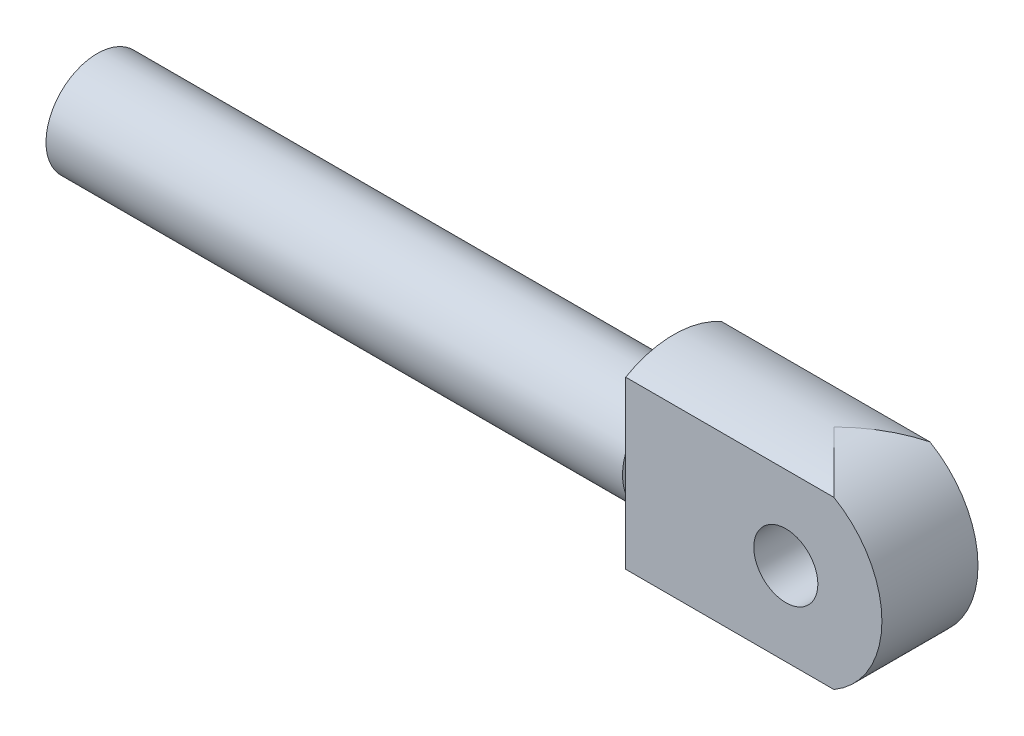
from build123d import *

# Parameters (mm, degrees)
BOSS_EXTRUDE1_START     = 100
SKETCH1_R               = 80
SKETCH1_R_2             = 50
BOSS_EXTRUDE1_DEPTH     = 900
BOSS_EXTRUDE2_DEPTH     = 400
CUT_EXTRUDE2_DEPTH      = 1417.518619715
CUT_EXTRUDE2_DEPTH_BACK = 1417.518619715
CUT_EXTRUDE3_DEPTH      = 1417.518619715
CUT_EXTRUDE3_DEPTH_BACK = 1417.518619715
SKETCH_4_5_2_R          = 50


with BuildPart() as part:
    # Sketch1 → Boss-Extrude1 (new body)
    with BuildSketch(Plane(origin=(0, 0, 0), x_dir=(0, 0, -1), z_dir=(1, 0, 0)).offset(BOSS_EXTRUDE1_START)):
        Circle(SKETCH1_R)
        Circle(SKETCH1_R_2, mode=Mode.SUBTRACT)
    extrude(amount=BOSS_EXTRUDE1_DEPTH)

    # Sketch3 → Boss-Extrude2 (add)
    with BuildSketch(Plane(origin=(1000, 0, 0), x_dir=(0, 0, -1), z_dir=(1, 0, 0))):
        with BuildLine():
            Line((-75, 129.903810568), (-75, -129.903810568))
            ThreePointArc((-75, -129.903810568), (0, -150), (75, -129.903810568))
            Line((75, -129.903810568), (75, 129.903810568))
            ThreePointArc((75, 129.903810568), (0, 150), (-75, 129.903810568))
        make_face()
    extrude(amount=BOSS_EXTRUDE2_DEPTH)

    # Sketch 4_5 → Cut-Extrude2 (cut, two sides: drawn at the far end of the back side and taken through both)
    with BuildSketch(Plane.XY.offset(75).offset(-CUT_EXTRUDE2_DEPTH_BACK)):
        with BuildLine():
            Line((1250, 150), (1455.357524725, 150))
            Line((1455.357524725, 150), (1455.357524725, -150))
            Line((1455.357524725, -150), (1250, -150))
            ThreePointArc((1250, -150), (1400, 0), (1250, 150))
        make_face()
    extrude(amount=CUT_EXTRUDE2_DEPTH + CUT_EXTRUDE2_DEPTH_BACK, mode=Mode.SUBTRACT)

    # Sketch 4_5 2 → Cut-Extrude3 (cut, two sides: drawn at the far end of the back side and taken through both)
    with BuildSketch(Plane.XY.offset(75).offset(-CUT_EXTRUDE3_DEPTH_BACK)):
        with Locations((1250, 0)):
            Circle(SKETCH_4_5_2_R)
    extrude(amount=CUT_EXTRUDE3_DEPTH + CUT_EXTRUDE3_DEPTH_BACK, mode=Mode.SUBTRACT)


solid = part.part
